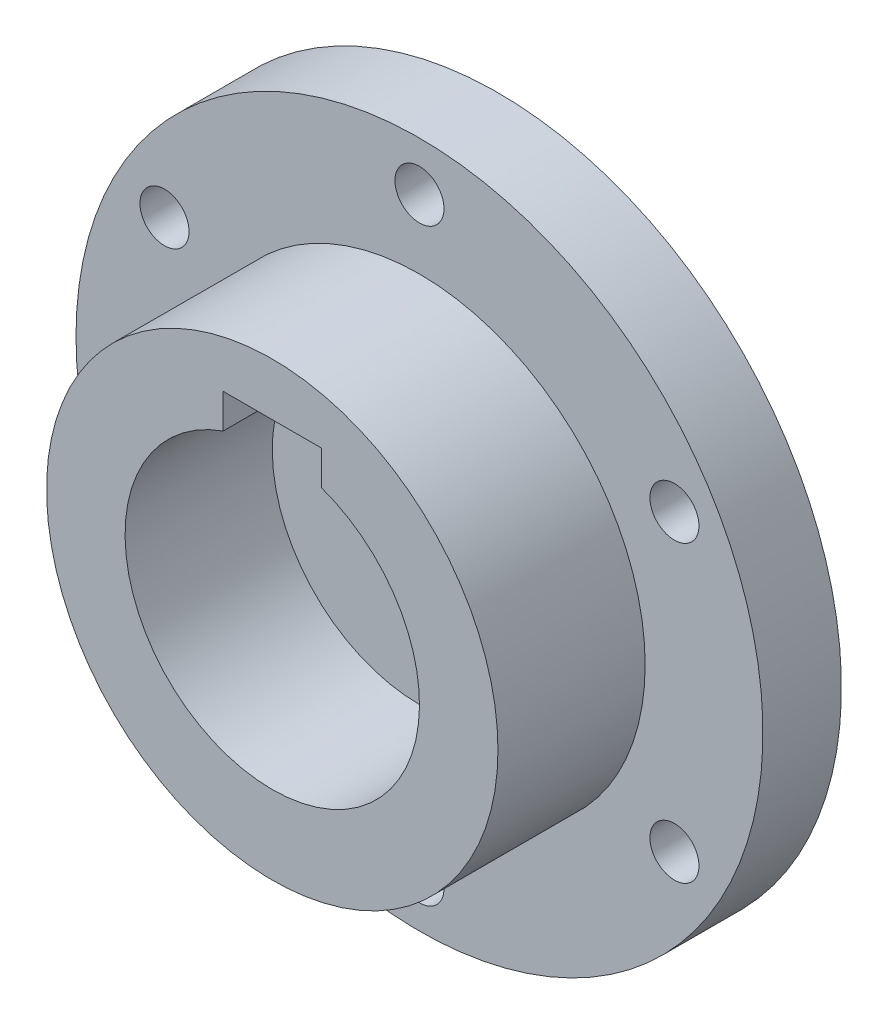
SolidWorks part; units mm, degrees
ref_plane "Front Plane" through (0, 0, 0) normal (0, 0, 1) x (1, 0, 0)
ref_plane "Top Plane" through (0, 0, 0) normal (0, 1, 0) x (1, 0, 0)
ref_plane "Right Plane" through (0, 0, 0) normal (1, 0, 0) x (0, 0, -1)
sketch "Sketch1" plane through (0, 0, 0) normal (0, 0, 1) x (1, 0, 0)
  line L0 (0, 298.7492) -> (0, -288.607) construction
  line L1 (-50, 141.4214) -> (-50, 176.4214)
  line L2 (-50, 176.4214) -> (50, 176.4214)
  line L3 (50, 141.4214) -> (50, 176.4214)
  arc A0 (-50, 141.4214) -> (50, 141.4214) centre (0, 0) ccw
  circle A1 centre (0, 0) radius 230
  point P9 (0, 176.4214)
  dimension "D1" = 300
  dimension "D4" = 460
  dimension "D2" = 50
  dimension "D3" = 35
extrude "Boss-Extrude1" add sketch "Sketch1" against normal blind 150
sketch "Sketch2" plane through (0, 0, -150) normal (0, 0, -1) x (-1, 0, 0)
  circle A0 centre (0, 0) radius 350
  dimension "D1" = 700
extrude "Boss-Extrude2" add sketch "Sketch2" along normal blind 80
sketch "Sketch3" plane through (0, 0, -230) normal (0, 0, -1) x (-1, 0, 0)
  circle A0 centre (0, 300) radius 25
  circle A1 centre (259.8076, 150) radius 25
  circle A2 centre (259.8076, -150) radius 25
  circle A3 centre (0, -300) radius 25
  circle A4 centre (-259.8076, -150) radius 25
  circle A5 centre (-259.8076, 150) radius 25
  point P16 (0, 0)
  dimension "D1" = 50
  dimension "D2" = 300
  dimension "D3" = 6
extrude "Cut-Extrude1" cut sketch "Sketch3" against normal blind 269 and the other way blind 256
cosmetic thread "Cosmetic Thread1" parameters "D2"=163.83
cosmetic thread "Cosmetic Thread2" parameters "D2"=163.83
cosmetic thread "Cosmetic Thread3" parameters "D2"=163.83
cosmetic thread "Cosmetic Thread4" parameters "D2"=163.83
cosmetic thread "Cosmetic Thread5" parameters "D2"=163.83
cosmetic thread "Cosmetic Thread6" parameters "D2"=163.83
